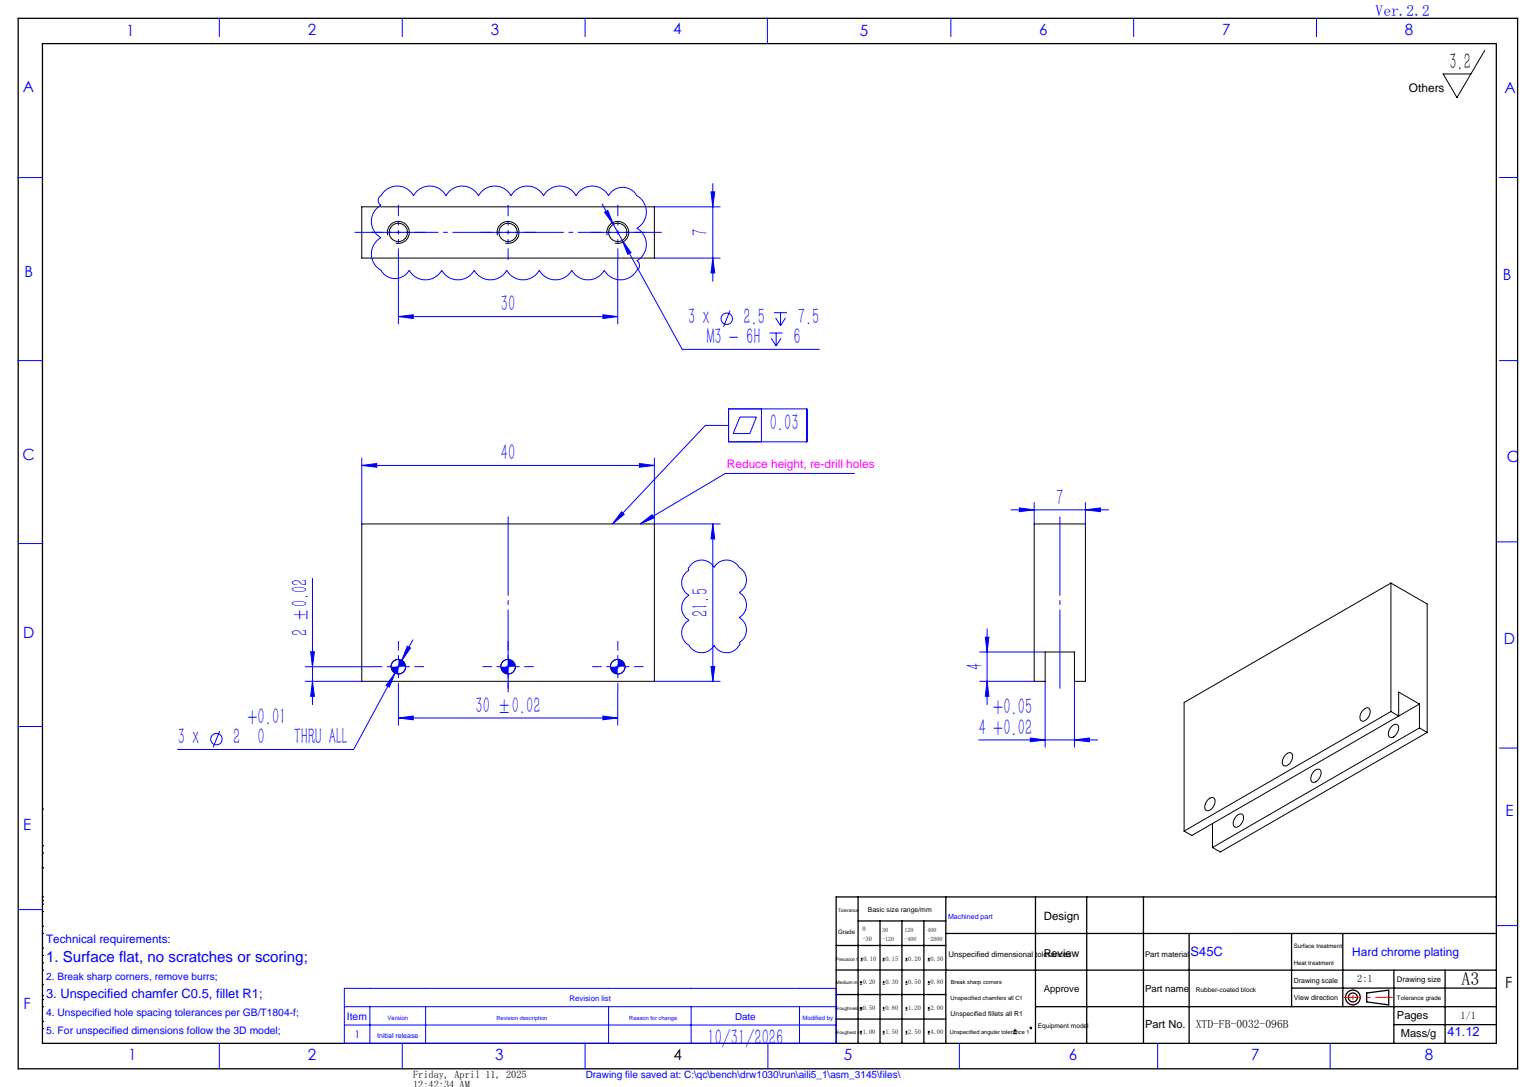
SolidWorks part; units mm, degrees
material "S45C"
ref_plane "前视基准面" through (0, 0, 0) normal (0, 0, 1) x (1, 0, 0)
ref_plane "上视基准面" through (0, 0, 0) normal (0, 1, 0) x (1, 0, 0)
ref_plane "右视基准面" through (0, 0, 0) normal (1, 0, 0) x (0, 0, -1)
sketch "草图1" plane through (0, 0, 0) normal (0, 0, 1) x (1, 0, 0)
  line L1 (-20, 3.5) -> (20, 3.5)
  line L2 (-20, 3.5) -> (-20, -3.5)
  line L3 (-20, -3.5) -> (20, -3.5)
  line L4 (20, 3.5) -> (20, -3.5)
  line L5 (-20, 3.5) -> (20, -3.5) construction
  line L6 (-20, -3.5) -> (20, 3.5) construction
  point P0 (0, 0)
  dimension "D1" = 40
  dimension "D2" = 7
extrude "凸台-拉伸1" add sketch "草图1" along normal blind 21.5
hole_wizard "M3 螺纹孔1" positions "草图2" profile "草图3" tap size "M3" standard "ISO"
sketch "草图2" plane through (0, 0, 21.5) normal (0, 0, 1) x (1, 0, 0)
  line L0 (0, 0) -> (0, -8.0132) construction
  line L1 (-20, 3.5) -> (-20, -3.5) construction
  point P0 (-15, 0)
  point P3 (0, 0)
  point P10 (15, 0)
  dimension "D1" = 5
sketch "草图3" plane through (-15, 0, 21.5) normal (1, 0, 0) x (0, -1, 0)
  line L0 (0, 0) -> (0, 8.2511)
  line L1 (0, 8.2511) -> (1.25, 7.5)
  line L2 (1.25, 7.5) -> (1.25, 0)
  line L5 (1.25, 0) -> (0, 0)
  line L10 (0, 8.2511) -> (-1.25, 7.5) construction
  line L11 (0, -6.35) -> (0, 107.95) construction
  dimension "螺纹孔钻头直径" = 2.5
  dimension "螺纹孔钻头深度" = 7.5
  dimension "导头角度" = 118
cosmetic thread "孔螺蚊线1" parameters "D1"=6, "D2"=3
cosmetic thread "孔螺蚊线2" parameters "D1"=6, "D2"=3
cosmetic thread "孔螺蚊线3" parameters "D1"=6, "D2"=3
sketch "草图4" plane through (20, 0, 0) normal (1, 0, 0) x (0, 0, -1)
  line L0 (0, -3.5) -> (0, 3.5) construction
  line L1 (-4, 2) -> (0, 2)
  line L2 (-4, 2) -> (-4, -2)
  line L3 (-4, -2) -> (0, -2)
  line L4 (0, 2) -> (0, -2)
  line L5 (-21.5, 0) -> (4.07, 0) construction
  line L6 (-21.5, -3.5) -> (-21.5, 3.5) construction
  dimension "D1" = 4
  dimension "D2" = 4
extrude "切除-拉伸1" cut sketch "草图4" against normal through all
hole_wizard "大小mm 暗销孔1" positions "草图5" profile "草图6" hole size "Ø2.0" standard "ISO" end condition through all
sketch "草图5" plane through (0, 3.5, 0) normal (0, 1, 0) x (1, 0, 0)
  point P0 (-15, -2)
  point P3 (0, -2)
  point P6 (15, -2)
sketch "草图6" plane through (-15, 3.5, 2) normal (1, 0, 0) x (0, 0, 1)
  line L0 (0, 0) -> (0, 7)
  line L1 (0, 7) -> (1, 7)
  line L2 (1, 7) -> (1, 0)
  line L5 (1, 0) -> (0, 0)
  line L11 (0, -6.35) -> (0, 107.95) construction
  dimension "通孔孔直径" = 2
  dimension "通孔孔深度" = 7
